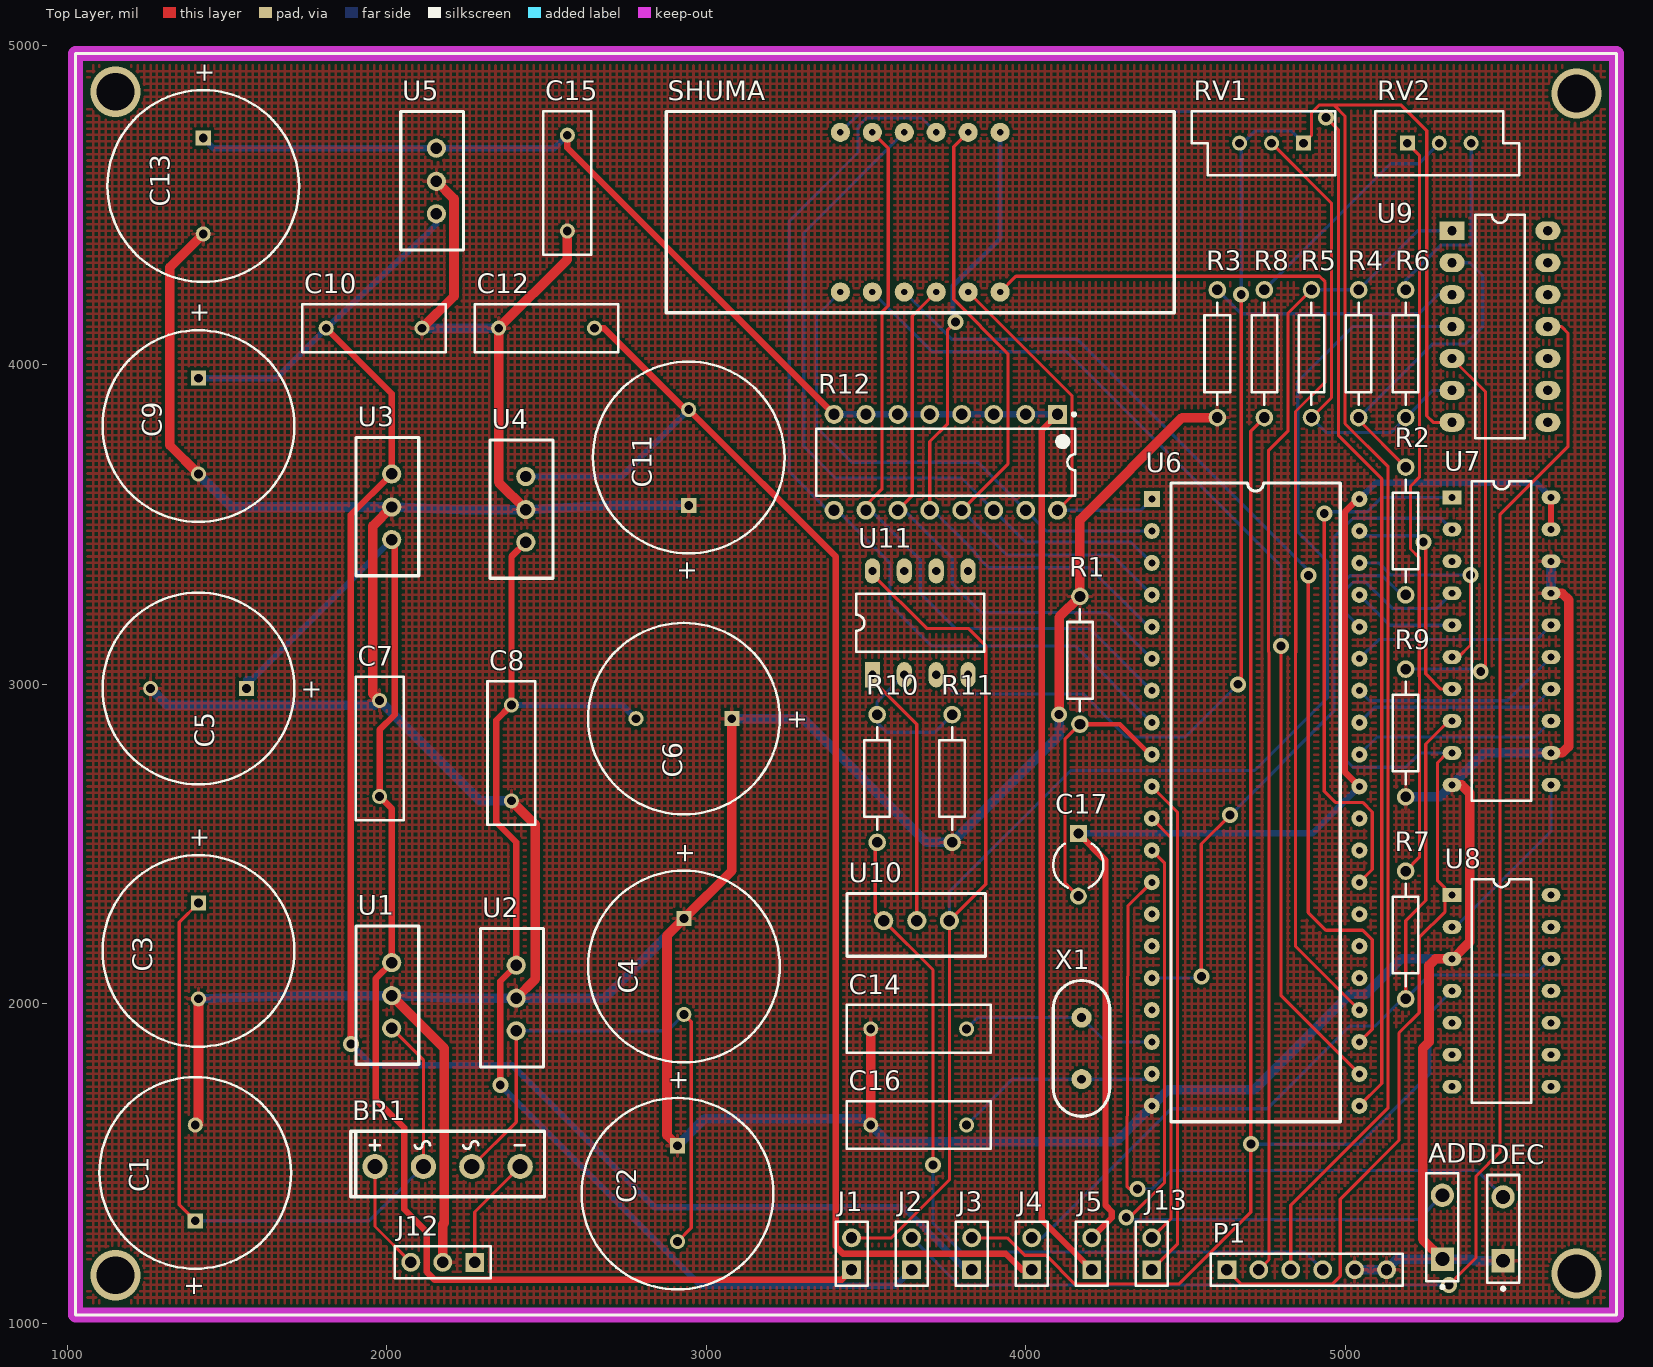
[diagram p0: Top Layer view]
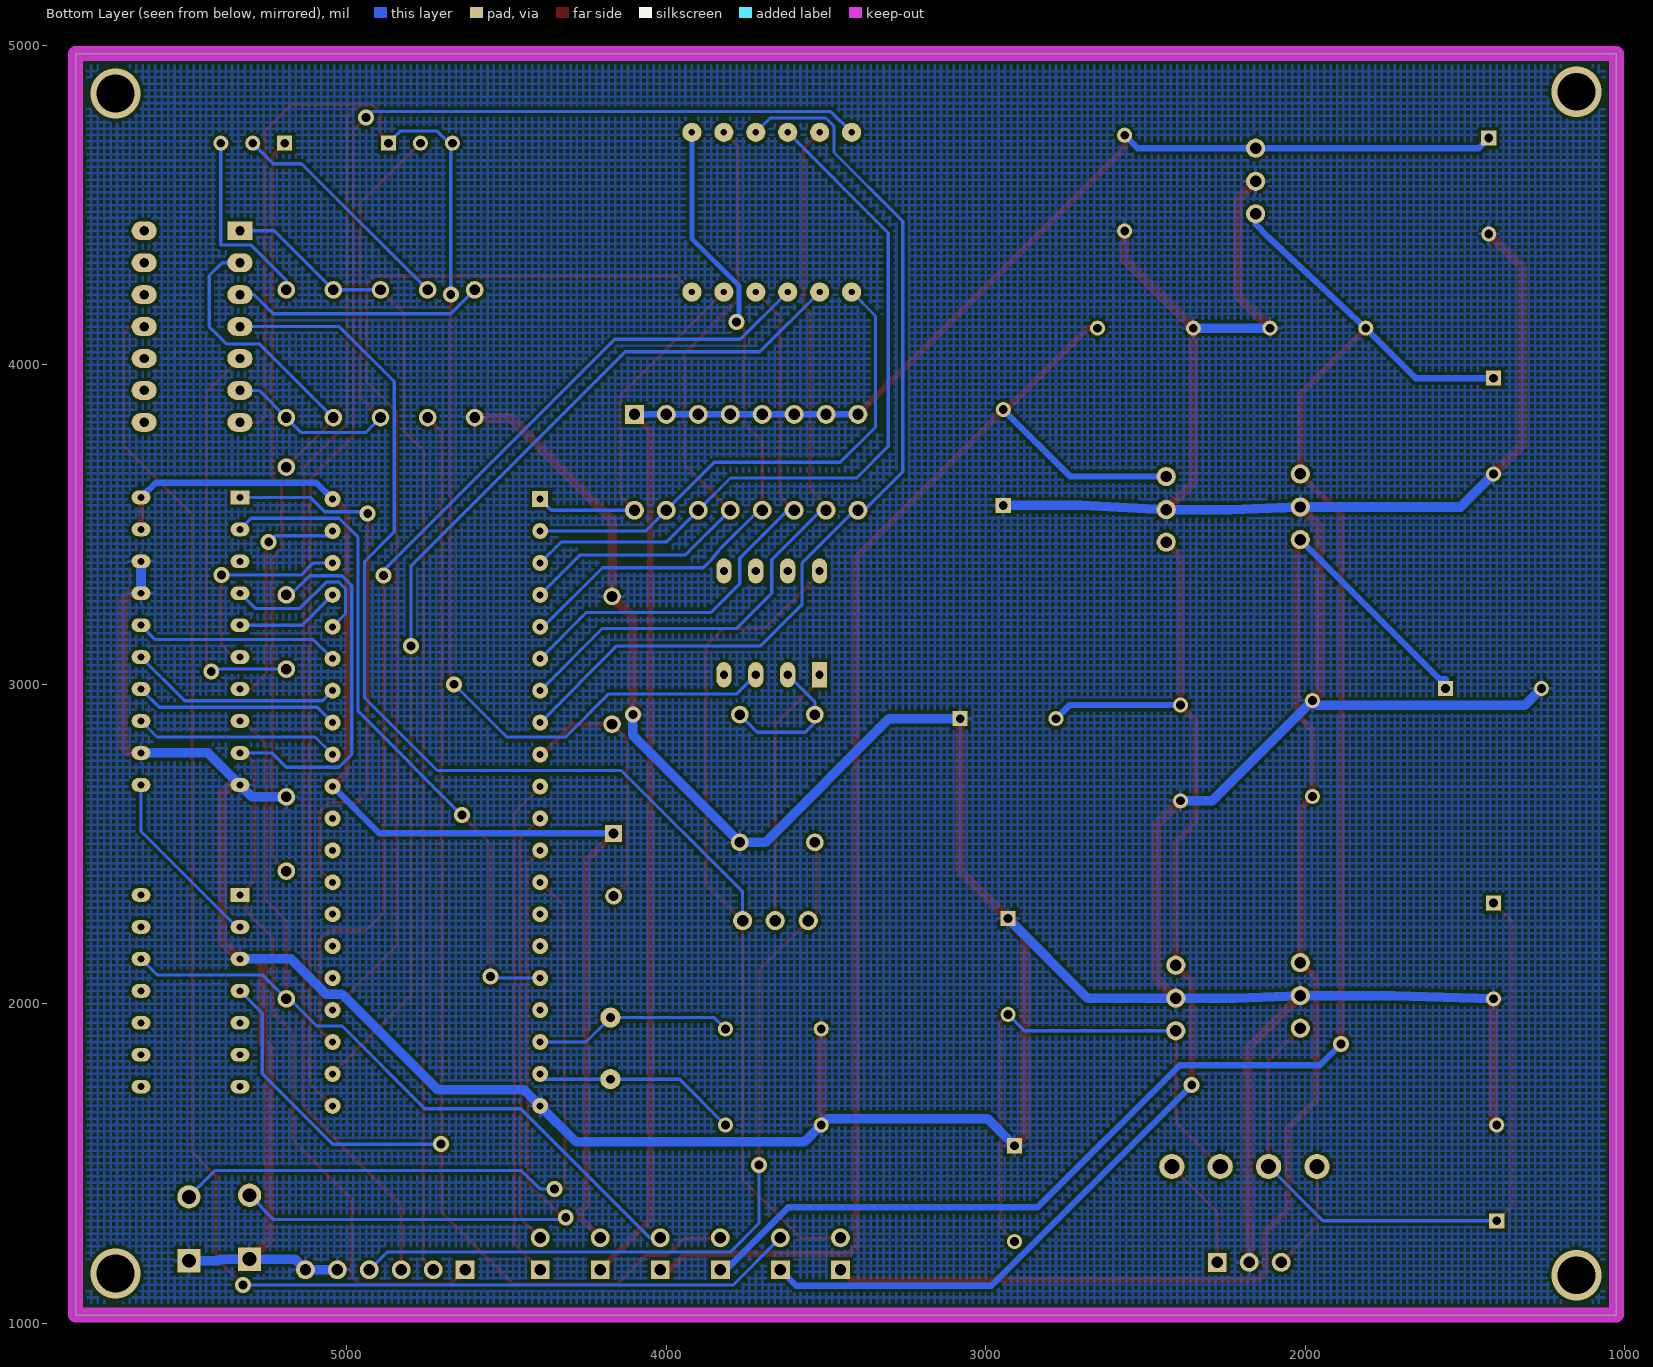
[diagram p1: Bottom Layer view, seen from below]
# Altium PCB MISC89340.PcbDoc
Units mil, origin at the board's own origin, x right, y up, seen from the top; angles counter-clockwise.
Board outline 4825 x 3950 mil, 2 copper layers (Top Layer, Bottom Layer); 55 components, 58 nets, 235 pads, 24 vias.

## Layer stack, top to bottom (the 12.6 mil dielectric is the usual default, probably not edited)
Top Solder: solder mask 0.4, Solder Resist, Dk 3.5
Top Layer: signal copper 1.4
Dielectric 1: dielectric 12.6, FR-4, Dk 4.8
Bottom Layer: signal copper 1.4
Bottom Solder: solder mask 0.4, Solder Resist, Dk 3.5

## Board outline
1025,1025 5850,1025 5850,4975 1025,4975

## Design rules (kind name [scope] priority, off if disabled: settings)
Clearance [All] p1: gap=10
HoleSize [All] p1: absolutevalues=TRUE maxlimit=500 minlimit=1 maxpercent=80.000 minpercent=20.000
PolygonConnect [All] p1: connectstyle=Relief reliefconductorwidth=10 reliefentries=4 polygonreliefangle="90 Angle" airgapwidth=10
RoomDefinition 智能稳压电源 [InComponentClass('智能稳压电源')] p1: confinementstyle=ConfineIn formatcopy=TRUE lockcomponents=FALSE outline 1015,1030 5860,1030 5860,4975 1015,4975
RoutingVias [All] p1: holewidth=28 width=50 viastyle="Through Hole" minholewidth=28 minwidth=50 maxholewidth=28 maxwidth=50
SilkToSolderMaskClearance [IsPad] p1: minsilkscreentomaskgap=0 clearancetoexposedcopper=TRUE
SolderMaskExpansion [All] p1: expansion=4
Width GND [InNet('T2')] p1: maxlimit=35 minlimit=20 preferedwidth=30
Width VCC [InNet('VCC')] p2: maxlimit=25 minlimit=10 preferedwidth=20
Width VCC_1 [InNet('+5V')] p3: maxlimit=25 minlimit=10 preferedwidth=20
Width VCC_2 [InNet('+9V')] p4: maxlimit=25 minlimit=10 preferedwidth=20
Width VCC_3 [InNet('+18V')] p5: maxlimit=25 minlimit=10 preferedwidth=20
Width VCC_4 [InNet('-9V')] p6: maxlimit=25 minlimit=10 preferedwidth=20
Width VCC_5 [InNet('-18V')] p7: maxlimit=25 minlimit=10 preferedwidth=20
Width [All] p8: maxlimit=15 minlimit=8 preferedwidth=10
28 further rules are at their usual default settings.

## Components (designator, comment, footprint, x,y, rotation, side; value= is the part's Value field where it differs from the comment)
ADD "SW-PB" SPST-2 5305,1300 r90 top
BR1 "Bridge1" LC-KBP 2190,1490 r0 top
C1 "Cap Pol1" RB7.6-15 1400,1470 r270 top
C2 "Cap Pol1" RB7.6-15 2910,1405 r90 top
C3 "Cap Pol1" RB7.6-15 1410,2165.14 r90 top
C4 "Cap Pol1" RB7.6-15 2930,2116.17 r90 top
C5 "Cap Pol1" RB7.6-15 1410,2986.76 r0 top
C6 "Cap Pol1" RB7.6-15 2930,2892.35 r0 top
C7 "Cap" RAD-0.3 1977.09,2798.94 r270 top
C8 "Cap" RAD-0.3 2390,2785 r270 top
C9 "Cap Pol1" RB7.6-15 1410,3808.38 r90 top
C10 "Cap" RAD-0.3 1960,4115 r180 top
C11 "Cap Pol1" RB7.6-15 2945,3710 r270 top
C12 "Cap" RAD-0.3 2500,4115 r180 top
C13 "Cap Pol1" RB7.6-15 1425,4560 r90 top
C14 "Cap" RAD-0.3 3665,1921.04 r0 top
C15 "Cap" RAD-0.3 2565,4569.13 r90 top
C16 "Cap" RAD-0.3 3665,1620 r0 top
C17 "Cap2" CAPR5-4X5 4165,2435 r270 top
DEC "SW-PB" SPST-2 5495,1295 r90 top
J1 "Header 2" HDR1X2 3455,1166.65 r90 top
J2 "Header 2" HDR1X2 3643,1166.65 r90 top
J3 "Header 2" HDR1X2 3831,1166.65 r90 top
J4 "Header 2" HDR1X2 4019,1166.65 r90 top
J5 "Header 2" HDR1X2 4207,1166.65 r90 top
J12 "Header 3" HDR1X3 2275,1190 r180 top
J13 "Header 2" HDR1X2 4395,1166.65 r90 top
P1 "Header 6" HDR1X6 4630,1166.65 r0 top
R1 "Res2" AXIAL-0.4 4170,3075 r270 top
R2 "Res2" AXIAL-0.4 5190,3480 r270 top
R3 "Res2" AXIAL-0.4 4600,4035 r270 top
R4 "Res2" AXIAL-0.4 5042.5,4035 r90 top
R5 "Res2" AXIAL-0.4 4895,4035 r90 top
R6 "Res2" AXIAL-0.4 5190,4035 r90 top
R7 "Res2" AXIAL-0.4 5190,2215 r270 top
R8 "Res2" AXIAL-0.4 4747.5,4035 r90 top
R9 "Res2" AXIAL-0.4 5190,2847.5 r270 top
R10 "Res2" AXIAL-0.4 3535,2705 r90 top
R11 "Res2" AXIAL-0.4 3770,2705 r270 top
R12 "Res Pack2" DIP-16 3750,3695 r270 top
RV1 "RPot" VR5 4770,4694.13 r180 top
RV2 "RPot" VR5 5295,4694.13 r0 top
SHUMA "Dpy Red-CA" 四位数码管 4465.28,4793.07 r180 top
U1 "7818" 7805 2100,1810 r90 top
U2 "7818" 7805 2490,1801.97 r90 top
U3 "7809" 7805 2100,3340 r90 top
U4 "7809" 7805 2520,3331.97 r90 top
U5 "7805" 7805 2240,4360 r90 top
U6 "89c51" 89c51 4395,3580 r0 top
U7 "Component_1" DAC0832 5335,3585 r0 top
U8 "Component_1" LM324 5335,2340 r0 top
U9 "Component_1" TL084 5335,4420 r0 top
U10 "7805" 7805 3874.13,2345 r180 top
U11 "" NE5532 3520,3029.8 r90 top
X1 "Component_1" LC-HC-49S 4175,1860 r90 top

## Footprints (in the part's own frame and the unit in brackets; to place one, negate y for a bottom-side part, rotate by r counter-clockwise, add the part's x,y. Pads: shape width x height; smd on the part's side, far side on the other; paste and mask are expansions set on the pad)
89c51 [mil]
  rect 50x50 hole 22: 1(0,0)
  round 50 hole 22: 2(0,-100) 3(0,-200) 4(0,-300) 5(0,-400) 6(0,-500) 7(0,-600) 8(0,-700) 9(0,-800) 10(0,-900) 11(0,-1000) 12(0,-1100) 13(0,-1200) 14(0,-1300) 15(0,-1400) 16(0,-1500) 17(0,-1600) 18(0,-1700) 19(0,-1800) 20(0,-1900) 21(650,-1900) 22(650,-1800) 23(650,-1700) 24(650,-1600) 25(650,-1500) 26(650,-1400) 27(650,-1300) 28(650,-1200) 29(650,-1100) 30(650,-1000) 31(650,-900) 32(650,-800) 33(650,-700) 34(650,-600) 35(650,-500) 36(650,-400) 37(650,-300) 38(650,-200) 39(650,-100) 40(650,0)
  silkscreen extent 60,-1950 590,50, body extent 65,-1950 590,55, height 190
7805 [mil]
  round 60 hole 35.83: 1(113.03,85) 2(215,85) 3(318.5,85)
  silkscreen extent 0,0 433,197
AXIAL-0.4 [mm] "Axial Device, Thru-Hole; 2 Leads; 0.4 in Pin Spacing"
  round 1.4 hole 0.85: 1(-5.08,0) 2(5.08,0)
  silkscreen extent -4.06,-1.02 4.06,1.02
CAPR5-4X5 [mm] "Capacitor; 2 Leads"
  rect 1.35x1.35 hole 0.8: 1(-2.5,0)
  round 1.35 hole 0.8: 2(2.5,0)
  silkscreen extent -1.69,-2 1.82,2
DAC0832 [mm]
  rect 1.5x1.1 hole 0.55: 1(0,0)
  oval 1.5x1.1 hole 0.55: 2(0,-2.54) 3(0,-5.08) 4(0,-7.62) 5(0,-10.16) 6(0,-12.7) 7(0,-15.24) 8(0,-17.78) 9(0,-20.32) 10(0,-22.86) 11(7.87,-22.86) 12(7.87,-20.32) 13(7.87,-17.78) 14(7.87,-15.24) 15(7.87,-12.7) 16(7.87,-10.16) 17(7.87,-7.62) 18(7.87,-5.08) 19(7.87,-2.54) 20(7.87,0)
  silkscreen extent 1.59,-24.13 6.29,1.27
DIP-16 [mm] "DIP; 16 Leads; Row Spacing 7.62 mm; Pitch 2.54 mm"
  rect 1.5x1.5 hole 0.9: 1(-3.81,8.89)
  round 1.5 hole 0.9: 2(-3.81,6.35) 3(-3.81,3.81) 4(-3.81,1.27) 5(-3.81,-1.27) 6(-3.81,-3.81) 7(-3.81,-6.35) 8(-3.81,-8.89) 9(3.81,-8.89) 10(3.81,-6.35) 11(3.81,-3.81) 12(3.81,-1.27) 13(3.81,1.27) 14(3.81,3.81) 15(3.81,6.35) 16(3.81,8.89)
  silkscreen extent -3.93,-10.3 2.65,10.32, body extent -3.6,-10.28 3.6,10.28, height 5.08
HDR1X2 [mm] "Connector; Header; 2 Position"
  rect 1.5x1.5 hole 0.9: 1(0,0)
  round 1.5 hole 0.9: 2(2.54,0)
  silkscreen extent -1.27,-1.27 3.81,1.27
HDR1X3 [mm] "Connector; Header; 3 Position"
  rect 1.5x1.5 hole 0.9: 1(0,0)
  round 1.5 hole 0.9: 2(2.54,0) 3(5.08,0)
  silkscreen extent -1.27,-1.27 6.35,1.27
HDR1X6 [mm] "Connector; Header; 6 Position"
  rect 1.5x1.5 hole 0.9: 1(0,0)
  round 1.5 hole 0.9: 2(2.54,0) 3(5.08,0) 4(7.62,0) 5(10.16,0) 6(12.7,0)
  silkscreen extent -1.27,-1.27 13.97,1.27
LC-HC-49S [mm]
  round 1.6 hole 0.7: 1(-2.45,0) 2(2.45,0)
  silkscreen extent -5.39,-2.25 5.39,2.25
LC-KBP [mm]
  round 2 hole 1.2: 1(-1.925,0) 2(-5.775,0) 3(1.925,0) 4(5.775,0)
  silkscreen extent -7.7,-2.4 7.7,2.8
LM324 [mm]
  rect 1.5x1.1 hole 0.55: 1(0,0)
  oval 1.5x1.1 hole 0.55: 2(0,-2.54) 3(0,-5.08) 4(0,-7.62) 5(0,-10.16) 6(0,-12.7) 7(0,-15.24) 8(7.87,-15.24) 9(7.87,-12.7) 10(7.87,-10.16) 11(7.87,-7.62) 12(7.87,-5.08) 13(7.87,-2.54) 14(7.87,0)
  silkscreen extent 1.59,-16.51 6.29,1.27
NE5532 [mm]
  rect 2x1.2 hole 0.65: 1(0,0)
  oval 2x1.2 hole 0.65: 2(0,-2.54) 3(0,-5.08) 4(0,-7.62) 5(8.26,-7.62) 6(8.26,-5.08) 7(8.26,-2.54) 8(8.26,0)
  silkscreen extent 1.84,-8.89 6.43,1.27
RAD-0.3 [mm] "Radial Cap, Thru-Hole; 2 Leads; 0.3 in Pin Spacing"
  round 1.2 hole 0.7: 1(-3.81,0) 2(3.81,0)
  silkscreen extent -5.72,-1.91 5.71,1.9
RB7.6-15 [mm] "Polarized Capacitor (Radial); 2 Leads"
  rect 1.2x1.2 hole 0.7: 1(3.81,0)
  round 1.2 hole 0.7: 2(-3.81,0)
  silkscreen extent -7.62,-7.62 7.62,7.62
SPST-2 [mm] "Switch; 2 Leads"
  rect 1.85x1.85 hole 1.1: 1(-2.54,0)
  round 1.85 hole 1.1: 2(2.54,0)
  silkscreen extent -4.89,-1.27 4.28,1.27
TL084 [mm]
  rect 2x1.5 hole 0.75: 1(0,0)
  oval 2x1.5 hole 0.75: 2(0,-2.54) 3(0,-5.08) 4(0,-7.62) 5(0,-10.16) 6(0,-12.7) 7(0,-15.24) 8(7.62,-15.24) 9(7.62,-12.7) 10(7.62,-10.16) 11(7.62,-7.62) 12(7.62,-5.08) 13(7.62,-2.54) 14(7.62,0)
  silkscreen extent 1.83,-16.51 5.79,1.27
VR5 [mm] "Thru-Hole; 3 Leads"
  rect 1.2x1.2 hole 0.7: 1(-2.54,0)
  round 1.2 hole 0.7: 2(0,0) 3(2.54,0)
  silkscreen extent -5.08,-2.54 6.35,2.54
四位数码管 [mm]
  round 1.524 hole 0.51: 1(13.85,1.65) 2(16.39,1.65) 3(18.93,1.65) 4(21.47,1.65) 5(24.01,1.65) 6(26.55,1.65) 7(26.55,14.35) 8(24.01,14.35) 9(21.47,14.35) 10(18.93,14.35) 11(16.39,14.35) 12(13.85,14.35)
  silkscreen extent 0,0 40.4,16

## Part data
ADD DEC: "Switch"
BR1: "Full Wave Diode Bridge"
C1 C2 C3 C4 C5 C6 C9 C11 C13: "Polarized Capacitor (Radial)"
C7 C8 C10 C12 C14 C15 C16 C17: "Capacitor"
J1 J2 J3 J4 J5 J13: "Header, 2-Pin"
J12: "Header, 3-Pin"
P1: "Header, 6-Pin"
R1 R2 R3 R4 R5 R6 R7 R8 R9 R10 R11: "Resistor"
R12: "Isolated Resistor Network - Parts"
RV1 RV2: "Potentiometer"
SHUMA: "7.62 mm Black Surface HER 7-Segment Display: CA, RH DP"
U1 U2 U3 U4 U5 U10: library part "Volt Reg", "Voltage Regulator"
U6 U11: library part Component_1

## Via types
v1: diameter 50, hole 28, Top Layer to Bottom Layer, 20 vias
v2: diameter 157.48, hole 118.11, Top Layer to Bottom Layer, 4 vias

## Nets (pads, with @x,y where several pads share a name; then routed paths per layer and width w, separated by ;. In a path a pad name is that pad's centre, name@x,y a point inside that pad or via, vN(x,y) a via of type N, cw(c..) or ccw(c..) an arc to the next point about the centre after c; other vN are vias at no path point)
1: SHUMA.12 U6.24 | length 3447.3
  Top Layer w10: SHUMA.12 3969.45,4277.56 4920,4277.56 4937.56,4260 4937.56,3946.56 4845,3854 4845,3323.43 4846,3322.43 4846,3099.43 4845,3098.43 4845,2180 U6.24
2: SHUMA.9 U6.23 | length 3269.6
  Top Layer w10: v1(4885,3340) 4885,2285 4940,2230 5055,2230 5085,2200 5085,1920 U6.23
  Bottom Layer w10: SHUMA.9 3768.11,4080 4162,4080 4885,3357 v1(4885,3340)
3: SHUMA.8 U6.22 | length 3326.9
  Top Layer w10: v1(4800,3120) 4800,2025 U6.22
  Bottom Layer w10: SHUMA.8 3707.11,4041 4129,4041 4800,3370 v1(4800,3120)
4: SHUMA.6 U6.21 | length 4750.9
  Top Layer w10: v1(4941,4774) 4979.94,4735.06 4979.94,3778.06 5115,3643 5115,1750 U6.21
  Bottom Layer w10: SHUMA.6 3485,4793.11 4921.89,4793.11 v1(4941,4774)
+5V: C13.1 C15.2 J5.1 R12.1 R12.2 R12.3 R12.4 R12.5 R12.6 R12.7 R12.8 U5.3 | length 5854
  Top Layer w20: C15.2 2565,4680 R12.8 ; R12.1 4050,3795 4050,1323.65 J5.1
  Bottom Layer w20: C13.1 1456.5,4678.5 U5.3 2524.37,4678.5 C15.2 ; R12.8 R12.7 R12.6 R12.5 R12.4 R12.3 R12.2 R12.1
+9V: C9.1 C10.2 J3.1 U3.3 U5.1 | length 5587.8
  Top Layer w20: C10.2 2015,3910 U3.3 1887,3530.5 v1(1887,1874)
  Bottom Layer w20: C9.1 1653.38,3958.38 C10.2 2115,4400 2155,4440 U5.1 ; v1(1887,1874) 1954,1807 2393,1807 2838,1362 3617.7,1362 3813.04,1166.65 J3.1
+18V: C5.1 C7.2 J1.1 U1.3 U3.1 | length 4437.6
  Top Layer w20: U3.1 2025,3443.03 2025,2905 1977.09,2857.09 C7.2 2015,2611.02 U1.3 1965,2078.5 1965,1700 2054,1611 2054,1356 2125,1285 2125,1160 2149,1136 3424.35,1136 J1.1
  Bottom Layer w20: C5.1 1560,3016 1577.97,3016 U3.1
+VDD: J1.2 U9.4 U10.1 U11.8 | length 5667.3
  Top Layer w10: J1.2 3580.03,1266.65 3761.1,1447.73 U10.1 3875,2373.9 3875,3120 3820,3175 3690,3175 3520,3345 U11.8
  Bottom Layer w10: U10.1 3761.1,2350.1 4141,2730 4717,2730 4945,2958 4945,3384 4852,3477 4852,3948 5024,4120 U9.4
+VEE: J3.2 R8.1 U8.4 | length 4472.8
  Top Layer w10: J3.2 3942,1266.65 3996.65,1212 4064,1212 4154,1122 4480,1122 4705,1347 v1(4705,1560) 4705,3792.5 R8.1
  Bottom Layer w10: v1(4705,1560) 5045,1560 5265,1780 5265,1970 U8.4
-9V: C11.2 C12.1 J4.1 U4.3 | length 4452.3
  Top Layer w20: C12.1 2680,4115 2935,3860 C11.2 3405,3400 3405,1240 3428,1217 3938,1217 3988.35,1166.65 J4.1
  Bottom Layer w20: U4.3 2735.47,3650.47 C11.2
-18V: C6.2 C8.1 J2.1 U2.3 U4.1 | length 3761.7
  Top Layer w20: v1(2355,1745) 2355,2070.47 U2.3 2405,2505 2342,2568 2342,2887 C8.1 2390,3400 U4.1
  Bottom Layer w20: v1(2355,1745) 2983,1117 3593.35,1117 J2.1 ; C8.1 2737.35,2935 C6.2
-VDD: J2.2 U9.11 | length 4949.9
  Top Layer w10: v1(5325,1119) 5410,1204.05 5410,1460 5485,1535 5485,3531 5698,3744 5698,4100 5678,4120 U9.11
  Bottom Layer w10: J2.2 3790.65,1119 v1(5325,1119)
-VEE: J4.2 R7.2 U7.8 U8.12 | length 2923.5
  Top Layer w10: R7.2 5190,2260 5253,2323 5253,2813 5325,2885 U7.8
  Bottom Layer w10: J4.2 4051.65,1266.65 4456.21,1671.21 4756.21,1671.21 5015,1930 5095,1930 5180,2015 R7.2 5265,2090 5594.84,2090 U8.12
A: R12.16 SHUMA.11 U6.1 | length 1145.9
  Top Layer w10: SHUMA.11 4145,3903.11 4145,3590 R12.16
  Bottom Layer w10: R12.16 4360,3545 U6.1
B: R12.15 SHUMA.7 U6.2 | length 1638.8
  Bottom Layer w10: SHUMA.7 3345,4153.11 3345,3805 3455,3695 3850,3695 R12.15 4065,3480 U6.2
C: R12.14 SHUMA.4 U6.3 | length 2354.8
  Bottom Layer w10: SHUMA.4 3305,4413.11 3305,3745 3404,3646 3799,3646 R12.14 4000,3445 4330,3445 U6.3
D: R12.13 SHUMA.2 U6.4 | length 2036.6
  Top Layer w10: R12.13 3944.53,3689.53 3944.53,4035.47 3775,4205 3775,4683.11 SHUMA.2
  Bottom Layer w10: R12.13 3940,3405 4270,3405 U6.4
D0: U6.39 U7.7 | length 732.3
  Top Layer w10: v1(5245,3445) 5245,3440 5252.56,3432.44 5252.56,3032.44 5300,2985 U7.7
  Bottom Layer w10: U6.39 5060,3465 5225,3465 v1(5245,3445)
D1: U6.38 U7.6 | length 656.5
  Top Layer w10: U7.6 5355,3085 5393,3123 v1(5393,3342)
  Bottom Layer w10: U6.38 5105,3380 5143,3342 v1(5393,3342)
D2: U6.37 U7.5 | length 329.4
  Bottom Layer w10: U6.37 5140,3185 U7.5
D3: U6.36 U7.4 | length 528.8
  Bottom Layer w10: U6.36 5005,3220 5005,3300 5025,3320 5065,3320 5147.56,3237.44 5287.44,3237.44 U7.4
D4: U6.35 U7.16 | length 643.3
  Bottom Layer w10: U6.35 5105,3140 5599.84,3140 U7.16
D5: U6.34 U7.15 | length 669.6
  Bottom Layer w10: U6.34 5076.65,2948.35 5508.19,2948.35 U7.15
D6: U6.33 U7.14 | length 643.3
  Bottom Layer w10: U6.33 5093.35,2928.35 5588.19,2928.35 U7.14
D7: U6.32 U7.13 | length 643.3
  Bottom Layer w10: U6.32 5100,2835 5594.84,2835 U7.13
DP: R12.9 SHUMA.3 U6.8 | length 2981.7
  Bottom Layer w10: SHUMA.3 3675,4773.11 3501.36,4773.11 3475,4746.75 3475,4665 3260,4450 3260,3665 3380,3545 R12.9 3410,3545 3575,3380 3575,3250 3705,3120 4155,3120 U6.8
E: R12.12 SHUMA.1 U6.5 | length 2148.6
  Top Layer w10: R12.12 3700,3760 3755.47,3815.47 3755.47,4110.47 v1(3780,4135) ; U6.5 U6.5@4395,3200
  Bottom Layer w10: R12.12 3710,3545 3830.69,3424.31 3858.62,3390.38 3884,3365 4200,3365 4385,3180 U6.5
  Bottom Layer w15: v1(3780,4135) 3772.5,4142.5 3772.5,4247.79 3920,4395.29 SHUMA.1
F: R12.11 SHUMA.10 U6.6 | length 1767.3
  Top Layer w10: R12.11 3645,3590 3645,4153.11 SHUMA.10
  Bottom Layer w10: R12.11 3620,3545 3770,3395 3770,3315 3860,3225 4250,3225 U6.6
G: R12.10 SHUMA.5 U6.7 | length 2423.4
  Top Layer w10: R12.10 3500,3560 3550,3610 3550,4165 3570,4185 3570,4678.11 SHUMA.5
  Bottom Layer w10: R12.10 3515,3545 3670,3390 3670,3285 3780,3175 4200,3175 U6.7
NetADD_2: ADD.2 U6.12 | length 2246.1
  Top Layer w10: v1(4315,1330) 4325,1330 4435,1440 4435,2440 U6.12
  Bottom Layer w10: v1(4315,1330) 4321,1324 5229,1324 ADD.2
NetBR1_1: BR1.1 C1.1 C3.1 U1.1 | length 2299.5
  Top Layer w10: C1.1 1350,1370 1350,2255.14 C3.1 ; U1.1 2114.21,1823.82 BR1.1
  Bottom Layer w10: C1.1 1944.21,1320 BR1.1
NetBR1_3: BR1.3 C2.2 C4.2 U2.1 | length 1767.4
  Top Layer w10: BR1.3 2405,1629.21 U2.1 ; C2.2 2953,1298 2953,1943.17 C4.2
  Bottom Layer w10: U2.1 2878.83,1915 C4.2
NetC14_2: C14.2 U6.18 X1.2 | length 626.3
  Bottom Layer w10: C14.2 3850.41,1956.46 X1.2 4251.46,1880 U6.18
NetC16_2: C16.2 U6.19 X1.1 | length 646.3
  Bottom Layer w10: C16.2 3958.54,1763.54 X1.1 4378.54,1763.54 U6.19
NetC17_2: C17.2 R1.2 U6.9 | length 839.6
  Top Layer w10: C17.2 4123,2378.57 4123,2828 R1.2
  Top Layer w15: R1.2 4295,2875 4390,2780 U6.9
NetDEC_2: DEC.2 U6.13 | length 2222.9
  Top Layer w10: v1(4350,1420) 4325,1420 4317,1428 4320.22,2305.76 U6.13
  Bottom Layer w10: v1(4350,1420) 4397,1420 4455,1478 5412,1478 DEC.2
NetR2_1: R2.1 R4.1 U9.2 | length 995.2
  Top Layer w10: R4.1 5042.5,3827.5 R2.1
  Bottom Layer w10: R4.1 5272.5,4065 5376,4065 5431,4120 5431,4280 5391,4320 U9.2
NetR3_1: R3.1 U9.3 | length 790.9
  Bottom Layer w10: R3.1 4675,4160 5231,4160 5291,4220 U9.3
NetR5_1: R5.1 R6.1 RV1.2 U9.6 | length 1476.9
  Top Layer w10: RV1.2 4957.56,4506.57 4957.56,3897.56 R5.1
  Bottom Layer w10: R5.1 4942,3788 5143,3788 R6.1 5275,3920 U9.6
NetR6_2: R6.2 RV2.3 | length 599.7
  Bottom Layer w10: R6.2 5190,4265 5300,4375 5395,4375 RV2.3
NetR7_1: R7.1 RV2.1 | length 2335.9
  Top Layer w10: R7.1 5233,2458 5233,3023.72 5232.56,3024.16 5232.56,3395.87 5205,3423.43 5205,3620 5233,3648 5233,4656.13 RV2.1
NetR8_2: R8.2 RV2.2 | length 737.7
  Bottom Layer w10: R8.2 5142.5,4630 5230.87,4630 RV2.2
NetR9_1: R9.1 U9.5 | length 1264.7
  Top Layer w10: U9.5 5440,3915 5440,3055 v1(5425,3040)
  Bottom Layer w10: R9.1 v1@5425,3047.5
NetR10_2: R10.2 R11.1 U11.2 | length 455.2
  Bottom Layer w10: U11.2 3535,2944.8 R10.2 3535,2880 3565,2850 3715,2850 R11.1
NetU7_11: U7.11 U8.2 | length 579.2
  Bottom Layer w10: U8.2 5345,2240 5644.84,2539.84 U7.11
NetU10_2: U10.2 U11.1 | length 819.4
  Top Layer w10: U11.1 3520,3014 3659.13,2874.87 U10.2@3659.13,2268
OUT: P1.3 RV1.1 RV1.3 U9.7 U11.3 | length 8374.2
  Top Layer w10: U11.3 U11.3@3720,3046 ; v1(4665,3000) 4675,3010 v1(4675,4220) ; P1.3 4830,1369 5135,1674 5135,3681 4999.94,3816.06 4999.94,4779.06 4965,4814 ; RV1.1 4895,4719.13 4895,4789 4920,4814 4965,4814 ; U9.7 5276,3820 5256,3840 5256,4733 5175,4814 4965,4814
  Bottom Layer w10: U11.3 3779.8,2970 4180,2970 4315,2835 4500,2835 v1(4665,3000) ; RV1.3 RV1.3@4675,4689.13 ; v1(4675,4220) RV1.3@4675,4689.13 ; RV1.1 4831.38,4732.76 4718.62,4732.76 RV1.3@4675,4689.13
OUT1: P1.1 R2.2 U7.9 U8.1 | length 3351.2
  Top Layer w10: P1.1 4674.65,1122 4960,1122 4985,1147 4985,1388 5169,1572 5169,1908.44 5232.56,1972 5232.56,2207.56 5313.21,2288.21 U8.1@5313.21,2330.21 ; U8.1 5290,2385 5290,2755 5320,2785 U7.9
  Bottom Layer w10: R2.2 5176.72,3280 5116.72,3340 5015.67,3340 4985,3309.33 4985,2780 5025,2740 5190,2740 5235,2785 U7.9
OUT2: P1.2 R4.2 R5.2 U9.1 | length 3655
  Top Layer w10: P1.2 4762,1198.65 4762,3101.43 4760,3103.43 4760,3731 4821,3792 4821,4161 R5.2
  Bottom Layer w10: R5.2 R4.2 5227.5,4420 U9.1
OUTPUT: P1.4 R10.1 U10.3 | length 2550.6
  Top Layer w10: R10.1 3529.02,2499.02 3529.02,2286.61 U10.3 3710,2105.63 v1(3710,1495)
  Bottom Layer w10: v1(3710,1495) 3710,1312 3800,1222 4874.65,1222 P1.4
P27: U6.28 U7.1 | length 1704.2
  Top Layer w10: v1(4935,3535) 4935,2665 4970,2630 5055,2630 5085,2600 5085,2420 U6.28
  Bottom Layer w10: v1(4935,3535) 4940,3540 5070,3540 5115,3585 U7.1
RXD: J13.1 U6.10 | length 1579.6
  Top Layer w10: J13.1 4475,1246.65 4475,2600 U6.10
T1: BR1.4 J12.1 | length 359
  Top Layer w10: J12.1 2275,1347.64 BR1.4
T2: ADD.1 C1.2 C2.1 C3.2 C4.1 C5.2 C6.1 C7.1 C8.2 C9.2 C10.1 C11.1 C12.2 C13.2 C14.1 C15.1 C16.1 DEC.1 J12.2 P1.5 P1.6 R1.1 R3.2 R9.2 R11.2 U1.2 U2.2 U3.2 U4.2 U5.2 U6.20 U7.10 U7.12 U7.17 U7.18 U8.3 | length 20074.3
  Top Layer w30: C1.2 1410,1630 C3.2 ; C9.2 1320,3748.38 1320,4305 C13.2 ; C7.1 1956,2970.02 1956,3496 U3.2 ; U1.2 2179,1861 2179,1313 2175,1309 J12.2 ; C10.1 2210,4215 2210,4520 U5.2 ; C8.2 2464,2561 2464,2075.97 U2.2 ; U4.2 2350,3631.97 C12.2 2565,4330 C15.1 ; C2.1 2877,1588 2877,2213.17 C4.1 3080,2416.17 C6.1 ; C16.1 C14.1 ; v1(4105,2905) 4105,3210 R1.1 4170,3515 4490,3835 R3.2 ; ADD.1 5243,1262 5243,1860 5263,1880 5263,2120 5283,2140 U8.3 ; U7.10 5365,2685 5390,2660 5390,2193 U8.3@5336,2139 ; U7.12 5680,2785 5700,2805 5700,3265 5680,3285 U7.17
  Bottom Layer w30: C5.2 1312.76,2934 1962.15,2934 C7.1 2291.02,2635 C8.2 ; C3.2 1722.86,2025 U1.2 2218.03,2016.97 U2.2 2680.79,2016.97 C4.1 ; C9.2 1513.38,3555 U3.2 2233.03,3546.97 U4.2 2703.03,3560 C11.1 ; C10.1 C12.2 ; C2.1 2995,1640 3495,1640 C16.1 3568,1567 4282,1567 U6.20 4445,1730 4715,1730 5015,2030 5065.71,2030 5175.71,2140 U8.3 ; C6.1 3302.65,2892.35 3690,2505 R11.2 4105,2840 v1(4105,2905) ; P1.5 P1.6 5163.35,1200 ADD.1 5397,1200 5402,1195 DEC.1 ; R9.2 5297.5,2647.5 U7.10 5435,2785 U7.12 ; U7.17 U7.18
T3: BR1.2 J12.3 | length 346.5
  Top Layer w10: BR1.2 1962.64,1302.36 J12.3
TXD: J13.2 U6.11 | length 1363.1
  Top Layer w10: J13.2 4455,1326.65 4455,2520 U6.11
VCC: C17.1 J5.2 U6.31 U6.40 U7.19 U7.20 | length 3957.3
  Top Layer w20: C17.1 4250,2448.43 4250,1368.64 4270,1348.64 4270,1329.65 J5.2 ; U6.31 5000,2725 5000,3540 5040,3580 U6.40 ; U7.19 U7.20
  Bottom Layer w20: C17.1 4898.43,2533.43 U6.31 ; U6.40 5096,3631 5598.84,3631 U7.20
WR: U6.16 U7.2 | length 2113.3
  Top Layer w10: v1(4550,2085) 4550,2500 v1(4640,2590)
  Bottom Layer w10: U6.16 4545,2080 v1(4550,2085) ; v1(4640,2590) 4965,2915 4965,3460 5025,3520 5300,3520 U7.2
pads on no net: U6.14 U6.15 U6.17 U6.25 U6.26 U6.27 U6.29 U6.30 U7.3 U8.5 U8.6 U8.7 U8.8 U8.9 U8.10 U8.11 U8.13 U8.14 U9.8 U9.9 U9.10 U9.12 U9.13 U9.14 U11.4 U11.5 U11.6 U11.7
copper on no net:
  other v2: 1150,1150 5725,1155 5725,4850 1150,4855

## Polygon pours and split planes (outlines as drawn)
T2 on Top Layer "Top Layer-No Net" (hatched 90Degree grid 20 track 8, pour order 0): 1025,4975 5860,4975 5860,1035 5850,1025 5845,1030 1025,1030
T2 on Bottom Layer "Top Layer-No Net" (hatched 90Degree grid 20 track 8, pour order 2): 1025,4960 5850,4960 5850,1025 1040,1025 1025,1040

## Keep-outs
Keep-Out Layer:
  the board outline again, w47.24

## Silkscreen, mask and mechanical layers (free items; w line width, h text height)
Top Overlay:
  the board outline again, w10